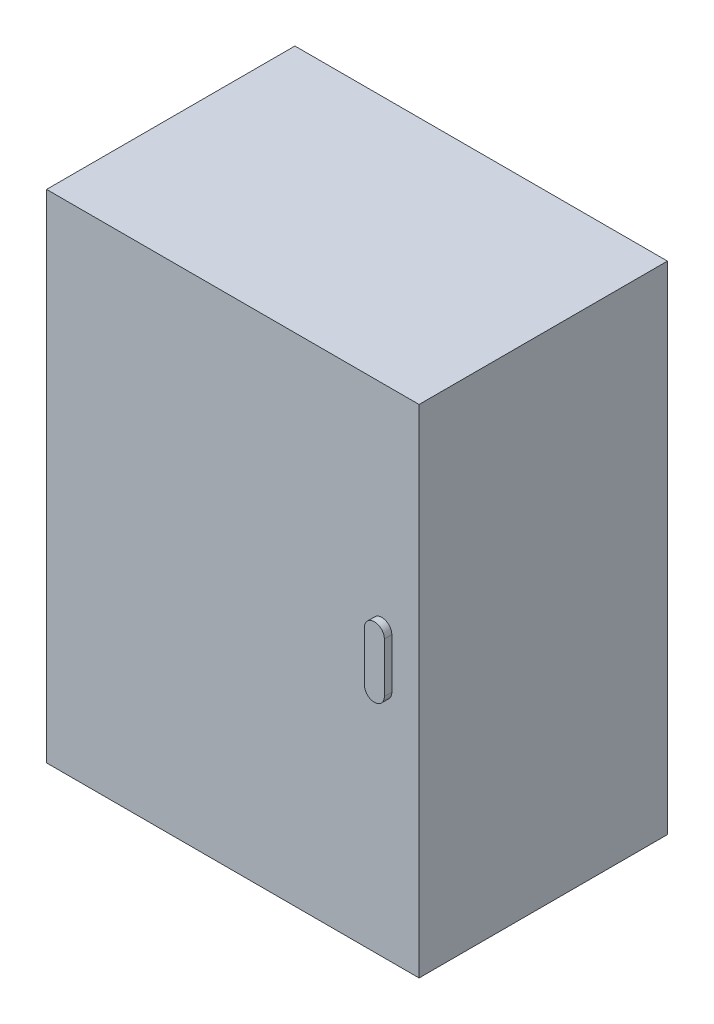
SolidWorks part; units mm, degrees
ref_plane "前视基准面" through (0, 0, 0) normal (0, 0, 1) x (1, 0, 0)
ref_plane "上视基准面" through (0, 0, 0) normal (0, 1, 0) x (1, 0, 0)
ref_plane "右视基准面" through (0, 0, 0) normal (1, 0, 0) x (0, 0, -1)
sketch "草图1" plane through (0, 0, 0) normal (0, 0, 1) x (1, 0, 0)
  line L1 (150, -200) -> (-150, -200)
  line L2 (150, -200) -> (150, 200)
  line L3 (150, 200) -> (-150, 200)
  line L4 (-150, -200) -> (-150, 200)
  line L5 (150, -200) -> (-150, 200) construction
  line L6 (150, 200) -> (-150, -200) construction
  point P0 (0, 0)
  dimension "D1" = 300
  dimension "D2" = 400
extrude "凸台-拉伸1" add sketch "草图1" along normal mid plane 200
sketch "草图2" plane through (0, 0, 100) normal (0, 0, 1) x (1, 0, 0)
  line L0 (120, 28.4542) -> (120, -11.6959) construction
  line L1 (128.03, 28.4542) -> (128.03, -11.6959)
  line L2 (111.97, 28.4542) -> (111.97, -11.6959)
  line L3 (150, -200) -> (150, 200) construction
  arc A0 (128.03, 28.4542) -> (111.97, 28.4542) centre (120, 28.4542) ccw
  arc A1 (111.97, -11.6959) -> (128.03, -11.6959) centre (120, -11.6959) ccw
  point P2 (120, 8.3792)
  dimension "D1" = 30
extrude "凸台-拉伸2" add sketch "草图2" along normal blind 6
